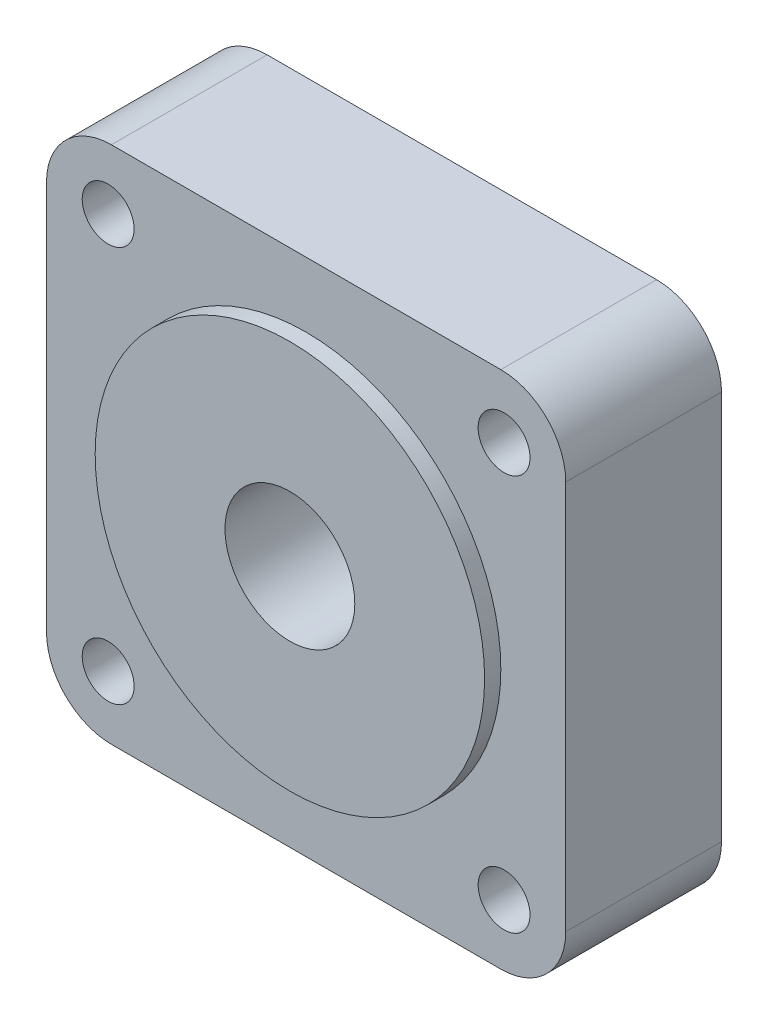
from build123d import *

# Parameters (mm, degrees)
SKETCH_1_W               = 80
SKETCH_1_H               = 80
EXTRUDE_1_DEPTH          = 24
FILLET_1_R               = 10
SKETCH_2_R               = 4
CUT_EXTRUDE_1_DEPTH      = 62.449165983
MIRROR_2_COPY_1_SKETCH_R = 4
MIRROR_2_COPY_1_DEPTH    = 62.449165983
SKETCH_3_R               = 30
EXTRUDE_2_DEPTH          = 2.5
SKETCH_4_R               = 10
CUT_EXTRUDE_2_DEPTH      = 49.5
CUT_EXTRUDE_3_DEPTH      = 2.5


with BuildPart() as part:
    # 草图1 → 凸台-拉伸1 (new body)
    with BuildSketch(Plane.XY):
        Rectangle(SKETCH_1_W, SKETCH_1_H)
    extrude(amount=EXTRUDE_1_DEPTH)

    # 圆角1
    fillet_1_edges = [part.edges().sort_by_distance(p)[0] for p in [
        (40, -40, 12),
        (-40, -40, 12),
        (-40, 40, 12),
        (40, 40, 12),
    ]]
    fillet(fillet_1_edges, radius=FILLET_1_R)

    # 草图2 → 切除-拉伸1 (cut, symmetric)
    with BuildSketch(Plane.XY.offset(24)):
        with Locations((-30.5, 30.5)):
            Circle(SKETCH_2_R)
    cut_extrude_1 = extrude(amount=CUT_EXTRUDE_1_DEPTH, both=True, mode=Mode.SUBTRACT)

    # 镜向1: 切除-拉伸1 across plane
    add(cut_extrude_1.mirror(Plane.ZX), mode=Mode.SUBTRACT)

    # 镜向2: 切除-拉伸1 across plane
    add(cut_extrude_1.mirror(Plane(origin=(0, 0, 0), x_dir=(0, 0, 1), z_dir=(1, 0, 0))), mode=Mode.SUBTRACT)

    # 镜向2 copy 1 sketch → 镜向2 copy 1 (cut, symmetric)
    with BuildSketch(Plane(origin=(0, 0, 24), x_dir=(-1, 0, 0), z_dir=(0, 0, 1))):
        with Locations((-30.5, 30.5)):
            Circle(MIRROR_2_COPY_1_SKETCH_R)
    extrude(amount=MIRROR_2_COPY_1_DEPTH, both=True, mode=Mode.SUBTRACT)

    # 草图3 → 凸台-拉伸2 (add)
    with BuildSketch(Plane.XY.offset(24)):
        with Locations(Location((0, 0, 0), (0, 0, 180))):
            Circle(SKETCH_3_R)
    extrude(amount=EXTRUDE_2_DEPTH)

    # 草图4 → 切除-拉伸2 (cut)
    with BuildSketch(Plane.XY.offset(26.5)):
        Circle(SKETCH_4_R)
    extrude(amount=-CUT_EXTRUDE_2_DEPTH, mode=Mode.SUBTRACT)

    # 草图5 → 切除-拉伸3 (cut)
    with BuildSketch(Plane(origin=(0, 0, 0), x_dir=(-1, 0, 0), z_dir=(0, 0, -1))):
        with BuildLine():
            Line((-23.263481458, -25.438517127), (23.263481458, -25.438517127))
            ThreePointArc((23.263481458, -25.438517127), (24.677695021, -24.852730689), (25.263481458, -23.438517127))
            Line((25.263481458, -23.438517127), (25.263481458, 23.438517127))
            ThreePointArc((25.263481458, 23.438517127), (24.677695021, 24.852730689), (23.263481458, 25.438517127))
            Line((23.263481458, 25.438517127), (-23.263481458, 25.438517127))
            ThreePointArc((-23.263481458, 25.438517127), (-24.677695021, 24.852730689), (-25.263481458, 23.438517127))
            Line((-25.263481458, 23.438517127), (-25.263481458, -23.438517127))
            ThreePointArc((-25.263481458, -23.438517127), (-24.677695021, -24.852730689), (-23.263481458, -25.438517127))
        make_face()
    extrude(amount=-CUT_EXTRUDE_3_DEPTH, mode=Mode.SUBTRACT)


solid = part.part
